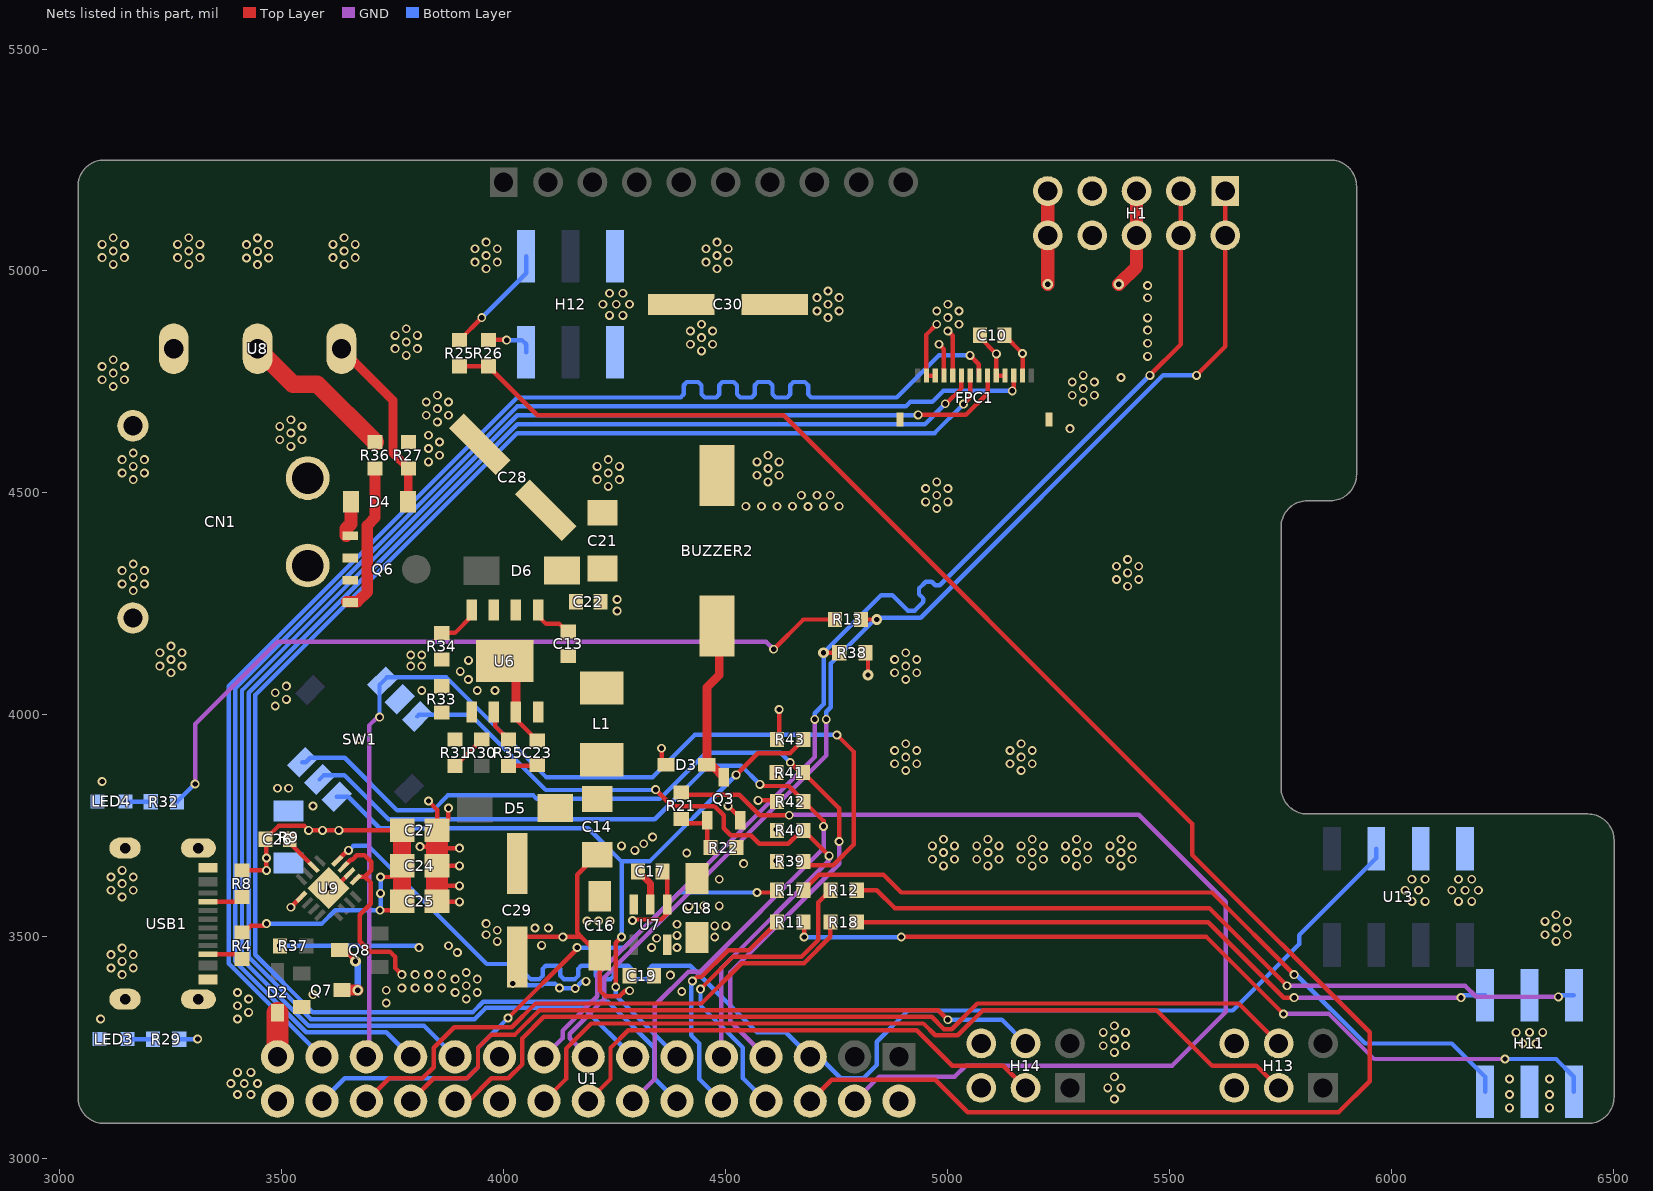
[diagram p0: the nets of this part, all layers, seen from the top]
# Altium PCB MISC51977.pcbdoc (part 2 of 4)
Units mil, origin at the board's own origin, x right, y up, seen from the top; angles counter-clockwise.
Board outline 3460 x 2170.19 mil, 4 copper layers (Top Layer, VCC, GND, Bottom Layer), stack 62.447 mil thick; 74 components, 60 nets, 282 pads, 462 vias.

## Via types
v1: diameter 20, hole 12, Top Layer to Bottom Layer, 455 vias
v2: diameter 24.02, hole 12, Top Layer to Bottom Layer, 7 vias

## Nets (pads, with @x,y where several pads share a name; then routed paths per layer and width w, separated by ;. In a path a pad name is that pad's centre, name@x,y a point inside that pad or via, vN(x,y) a via of type N, cw(c..) or ccw(c..) an arc to the next point about the centre after c; other vN are vias at no path point)
3V3: C10.2 C18.1 C19.1 FPC1.4 FPC1.10 FPC1.11 H1.5 H1.6 H1.9 H1.10 H13.5 H14.5 R13.2 R32.1 R38.2 R39.1 R40.1 R41.2 R42.2 R43.2 U7.5 | length 2550.2
  Top Layer w10: v1(4572.5,3807.5) 4611.88,3807.5 R42.2@4613.15,3808.77 ; v1(4607.56,4147.94) 4674.62,4215 R13.2@4745.34,4215 ; R43.2@4613.15,3941.94 4620.34,3949.13 4620.34,4012.78 v1(4620,4012.44) ; R38.2@4814.66,4140 4820,4134.66 v2(4820,4090) ; v1(4980,4835) 4991.1,4823.9 FPC1.4@4991.1,4764.22 ; C10.2@5072.44,4855 5072.44,4850 v1(5109.22,4813.23) FPC1.10@5109.22,4764.22 FPC1.11@5128.9,4764.22
  Top Layer w30: v2(5225,4970) H1.10@5225,5080 H1.9@5225,5180 ; v2(5385,4970) 5425,5010 H1.6@5425,5080 H1.5@5425,5180
  GND w10: v1(3304.54,3844.54) 3304.54,3979.54 3490,4165 4590.5,4165 v1(4607.56,4147.94)
  Bottom Layer w10: R32.1@3263.73,3804.54 3303.73,3844.54 v1(3304.54,3844.54)
  other v1: 4400.56,3376.99 4375,3414.02 4332.74,3475.98 4390,3475.98 4343.96,3497.01 4475,3500 4390,3503.59 4475,3525 4500,3525 4390,3528.56 4613.15,3671.94 4613.15,3741.94 4615,3866.94 5275,4645 5305,4705 5280,4720 5330,4720 5305,4735 5280,4750 5330,4750 5305,4765
$1N4144: CN1.2 D4.1 Q6.1 Q6.2 Q6.3 U8.3 | length 79.4
  Top Layer w30: Q6.1@3645.11,4405 3645.11,4420.11 3655.63,4430.63 D4.1@3655.63,4480
$1N4169: D4.2 R27.2 U8.1 | length 407.8
  Top Layer w20: U8.1@3633.97,4825 3750,4708.98 3750,4590.34 R27.2@3785,4555.34 3784.37,4554.71 D4.2@3784.37,4480
$1N4273: H11.2 R12.1 | length 1713.9
  Top Layer w10: R12.1@4794.66,3605.05 4839.95,3605.05 4880,3565 5589.02,3565 v1(5764.02,3390)
  GND w10: v1(5764.02,3390) 6165,3390 6190,3365 v1(6375,3365)
  Bottom Layer w10: v1(6375,3365) v1@6376.73,3363.27 ; v1@6378.27,3368.27 H11.2@6410,3368.27
$1N4282: R4.1 USB1.10 | length 80.9
  Top Layer w10: USB1.10@3333.51,3461.09 3399.24,3461.09 R4.1@3410,3450.34
$1N4283: R8.1 USB1.4 | length 80.9
  Top Layer w10: USB1.4@3333.51,3579.2 3399.34,3579.2 R8.1@3410,3589.87
$1N4817: BUZZER2.2 D3.2 Q3.3 | length 368.8
  Top Layer w20: BUZZER2.2@4485,4192.82 4485,4090 4457.38,4062.38 4457.38,3882.89 4472.1,3882.89 Q3.3@4495.26,3859.73
$1N4974: Q3.1 R21.2 R22.1 | length 120.6
  Top Layer w10: R21.2@4399.34,3755.8 4451.19,3755.8 Q3.1@4457.86,3762.48 4457.86,3713.16 R22.1@4464.92,3706.1
$1N5665: Q7.3 Q8.3 | length 146
  Top Layer w15: Q8.3@3635.63,3470 3644.48,3470 3665.69,3448.79 v2(3665.69,3445.39)
  Top Layer w25: Q7.3@3634.37,3380 v2(3670.69,3380)
  Bottom Layer w15: v2(3665.69,3445.39) 3670.69,3440.39 v2(3670.69,3380)
$1N14385: H11.1 R11.2 | length 1932
  Top Layer w10: R11.2@4674.66,3533.35 4676.3,3531.71 v1(4676.3,3499.64) ; v1(4895,3500) 5582.46,3500 v1(5755.98,3326.47)
  GND w10: v1(5755.98,3326.47) 5858.53,3326.47 5960,3225 v1(6255,3225)
  Bottom Layer w10: v1(4676.3,3499.64) 4894.64,3499.64 v1(4895,3500) ; v1(6255,3225) 6370,3225 6410,3185 H11.1@6410,3151.73
$1N14395: H11.6 R18.1 | length 1480.8
  Top Layer w10: R18.1@4794.66,3533.35 5586.65,3533.35 5756.73,3363.27 v1(5780,3363.27)
  GND w10: v1(5780,3363.27) v1(6155.98,3363.27)
  Bottom Layer w10: v1@6160.98,3368.27 H11.6@6210,3368.27
$1N14409: H11.5 R17.2 | length 1771.6
  Top Layer w10: R17.2@4674.66,3605.05 4709.61,3640 4855,3640 4895,3600 5595,3600 v1(5780,3415)
  Bottom Layer w10: v1(5780,3415) 5785,3415 5940,3260 6135,3260 6210,3185 H11.5@6210,3151.73
$1N22821: R36.1 U8.2 | length 352.1
  Top Layer w40: U8.2@3445,4825 3524.99,4745 3579.66,4745 R36.1@3710,4614.66
$1N23425: C26.1 U9.6 | length 85.1
  Top Layer w10: C26.1@3517.56,3720 3517.56,3711.36 U9.6@3571.59,3657.32
$1N29256: LED3.2 R29.1 | length 57.4
  Bottom Layer w10: LED3.2@3152.17,3269.92 3209.03,3269.92 R29.1@3209.41,3269.54
$1N41370: Q6.4 R36.2 | length 341.8
  Top Layer w25: Q6.4@3645.11,4255 3670,4255 3692.14,4277.14 3692.14,4427.14 3710,4445 R36.2@3710,4555.34
$1N45237: H12.6 R25.1 | length 250.7
  Top Layer w10: R25.1@3900,4844.66 3950,4894.66 v1(3950,4895)
  Bottom Layer w10: v1(3950,4895) 4050,4995 H12.6@4050,5033.27
$1N45238: H12.5 R26.1 | length 107.3
  Top Layer w10: R26.1@3965,4844.66 4005.77,4844.66 v1(4006.06,4844.37)
  Bottom Layer w10: v1(4006.06,4844.37) 4040.63,4844.37 4050,4835 H12.5@4050,4816.73
$2N1741: R34.2 U6.4 | length 96.4
  Top Layer w10: R34.2@3860,4184.66 3889.66,4184.66 3927.11,4222.11 U6.4@3927.11,4235.93
$2N1742: C21.2 C22.2 C28.1 D6.2 U6.2 U6.3
$2N1743: C13.2 U6.1 | length 95.6
  Top Layer w10: U6.1@4077.11,4235.93 4077.11,4222.89 4095,4205 4125,4205 4142.44,4187.56 C13.2@4145,4187.56
$2N1744: C13.1 L1.1 U6.8
$2N1746: C23.2 R35.1 | length 65.9
  Top Layer w10: R35.1@4010,3885.34 4072.9,3885.34 C23.2@4075,3887.44
$2N1747: R35.2 U6.6 | length 75.9
  Top Layer w10: U6.6@3977.11,4006.93 3980,4004.04 3980,3975 4010,3945 R35.2@4010,3944.66
$2N1748: R31.1 R33.2 U6.5
$2N1752: C14.2 C29.1 D5.1 L1.2
$2N1753: R30.1 R31.2 | length 84.6
  Top Layer w10: R31.2@3890,3885.34 3890.68,3885.34 R30.1@3950,3944.66
$2N1757: LED4.2 R32.2 | length 57.4
  Bottom Layer w10: LED4.2@3147.17,3804.92 3147.54,3804.54 R32.2@3204.41,3804.54
+5V: BUZZER2.1 C16.1 C17.1 C24.1 C25.1 C27.2 C30.1 D2.1 D3.1 Q7.2 R29.2 U1.29 U7.1 U7.3 U9.1 U9.3 U9.9 U13.7 | length 1386.8
  Top Layer w10: v1@3520,3565 v1(3520,3566.75) U9.9@3543.75,3590.51 ; U9.3@3638.36,3657.37 3655.01,3674.02 3658.69,3674.02 3668.69,3684.02 3685.98,3684.02 3700.86,3669.14 3700.86,3650.05 3686.67,3635.86 ; U9.1@3665,3629.53 U9.1@3666.2,3629.53 3672.53,3635.86 3686.67,3635.86 ; v1(3770,3415) 3755,3430 3755,3455 3742.93,3467.07 3697.93,3467.07 3675,3490 3675,3550 3700,3575 3700,3622.53 3686.67,3635.86 ; v1(3811,3703.43) 3848.37,3703.43 3849.37,3704.43 ; v1(3830,3805.98) 3849.37,3786.61 C27.2@3849.37,3740 3875,3765.63 v1(3875,3790) ; C25.1@3849.37,3580 3850.39,3578.98 v1(3900,3578.98) ; 3849.37,3615 v1(3900,3615) ; C24.1@3849.37,3660 v1(3900,3660) ; 3849.37,3710.63 3860,3700 v1(3900,3700) ; v1(4289.6,3536.98) 4291.9,3539.28 4354.28,3539.28 4367.4,3552.4 U7.1@4367.4,3573.04 4367.4,3637.78 C17.1@4357.56,3647.62 ; v1(4355,3925) 4355,3897.95 D3.1@4365.05,3887.89
  Top Layer w50: U1.29@3490,3230 D2.1@3490,3328.84 ; C25.1@3849.37,3580 3849.37,3615 C24.1@3849.37,3660 3849.37,3704.43 3849.37,3710.63 C27.2@3849.37,3740
  Bottom Layer w10: R29.2@3268.73,3269.54 3269.19,3270 v1(3310,3270)
  other v1: 3400,3315 3425,3330 3400,3345 3735,3350.98 3425,3360 3915,3360 3570,3370 3400,3375 3890,3375 3940,3375 3735,3380 3770,3385 3800,3385 3830,3385 3860,3385 3915,3390 3890,3405 3940,3405 3800,3415 3830,3415 3860,3415 3915,3420 4187.46,3536.06 4213.41,3536.06 4238.56,3536.06 6150,3580 6180,3580 6135,3605 6165,3605 6195,3605 6150,3630 6180,3630 4545,4470 4580,4470 4615,4470 4650,4470 4685,4469.59 4720,4470 4755,4470 4670,4495 4705,4495 4735,4495 4595,4525 4570,4540 4620,4540 4595,4555 4570,4570 4620,4570 4595,4585 4445,4820 4420,4835 4470,4835 4445,4850 4420,4865 4470,4865 4445,4880
AGND: C24.2 C25.2 C26.2 C27.1 R4.2 R8.2 R9.1 U9.2 U9.17 | length 1171.1
  Top Layer w10: R4.2@3410,3509.66 3414.66,3509.66 3430,3525 3460,3525 v1(3465,3530) ; R8.2@3410,3649.19 3410.81,3650 v1(3465,3650) v1(3465,3677.66) 3465,3717.44 C26.2@3462.44,3720 3492.44,3750 3550,3750 v1(3560,3740) v1(3591.39,3740) v1(3628.21,3740) C27.1@3770.63,3740 ; U9.17@3624.99,3610.01 3624.99,3616.15 U9.2@3652.28,3643.44 ; v1(3720.98,3560) 3750.63,3560 C25.2@3770.63,3580 ; v1(3722.15,3635) 3767.14,3635 3770.63,3631.51
  Top Layer w40: C25.2@3770.63,3580 3770.63,3631.51 C24.2@3770.63,3660 C27.1@3770.63,3740
  Bottom Layer w10: v1(3465,3530) 3590,3530 3620,3560 v1(3720.98,3560) 3722.15,3561.16 v1(3722.15,3598.06) v1(3722.15,3635)
  other v1: 3604.99,3610
BUZZER: R21.1 U1.4 | length 2496.7
  Top Layer w10: R21.1@4399.34,3815.12 4404.22,3820 4530,3820 4576,3774 v1(4642.81,3774)
  GND w10: v1(4642.81,3774) 4643.81,3775 5430,3775 5626.09,3578.91 5626.09,3331.09 5505,3210 5040,3210 5015,3185 4845,3185 U1.4@4790,3130
ENCODER_DIR_L: H13.3 U1.18 | length 1874.6
  Top Layer w10: U1.18@4090,3130 4140,3180 4140,3248.43 4196.57,3305 4945,3305 4971.69,3278.31 5022.41,3278.31 5079.11,3335 5470,3335 5595,3210 5695,3210 H13.3@5745,3160
ENCODER_DIR_R: H14.3 U1.16 | length 1146.1
  Top Layer w10: U1.16@4190,3130 4240,3180 4240,3250 4280,3290 4930,3290 5010,3210 5125,3210 H14.3@5175,3160
ENCODER_PWM_L: H13.4 U1.22 | length 2040.6
  Top Layer w10: U1.22@3890,3130 3920,3130 3971.61,3181.61 4010.04,3181.61 4041.61,3213.19 4041.61,3271.61 4090,3320 4963.63,3320 4991.31,3292.32 5008.69,3292.32 5066.37,3350 5655,3350 H13.4@5745,3260
ENCODER_PWM_R: H14.4 U1.24 | length 1526.4
  Top Layer w10: U1.24@3790,3130 3841.61,3181.61 3916.61,3181.61 3941.61,3206.61 3941.61,3250.04 3971.57,3280 4025,3280 4080,3335 4978.31,3335 v1(5000,3313.31)
  Bottom Layer w10: v1(5000,3313.31) 5121.69,3313.31 H14.4@5175,3260
GND: C10.1 C14.1 C16.2 C17.2 C18.2 C19.2 C21.1 C22.1 C23.1 C28.2 C29.2 C30.2 CN1.1 CN1.3 CN1.4 FPC1.2 FPC1.3 FPC1.5 FPC1.13 FPC1.15 FPC1.16 H1.7 H1.8 H11.3 H11.4 H12.1 H12.2 H13.6 H14.6 LED3.1 LED4.1 Q3.2 R9.2 R22.2 R27.1 R33.1 R34.1 R37.1 SW1.2 U1.2 U1.19 U1.20 U1.30 U6.7 U6.9 U7.2 U13.5 USB1.1 USB1.12 USB1.13 USB1.14 | length 1810.8
  Top Layer w10: v1(3495,3480) R37.1@3495.34,3480 R37.1@3495.68,3479.66 ; U6.7@4027.11,4006.93 4027.11,3990.45 C23.1@4075,3942.56 ; C29.2@4030,3449.88 4030,3500 v1(4132.83,3500) 4174.1,3500 ; C14.1@4210.19,3685.13 4165,3639.94 4165,3509.1 4174.1,3500 ; v1(4283.22,3378.65) 4273,3378.65 4260.52,3366.17 4228.83,3366.17 4215.49,3379.51 C16.2@4215.49,3458.61 4174.1,3500 ; v1(4505,3795) 4532.66,3767.34 Q3.2@4532.66,3762.48 ; FPC1.3@4971.41,4764.22 FPC1.2@4951.73,4764.22 4951.73,4856.73 v1(4975,4880) ; v1(5000,4865) 5010.78,4854.22 FPC1.5@5010.78,4764.22 ; C10.1@5127.56,4855 v1(5168.27,4814.3) FPC1.13@5168.27,4764.22
  Top Layer w15: C17.2@4302.44,3647.62 4330,3620.06 U7.2@4330,3573.04
  Top Layer w20: U6.9@4002.11,4121.43 4027.11,4096.43 U6.7@4027.11,4006.93
  Bottom Layer w10: v1(3495,3480) 3804.68,3480 v1(3808.82,3475.86) ; v1(4020,3395) 4050.18,3395 4054.19,3390.98 4085.81,3390.98 4089.82,3395 4115,3395 v1(4125,3385) 4125.98,3384.02 v1(4160.51,3384.02) 4176.5,3400 v1(4185,3400)
  other v1: 6265,3115 6355,3115 5375,3135 3400,3145 3430,3145 6265,3145 6355,3145.1 5360,3160 5390,3160 3385,3170 3415,3170 3445,3170 6265,3180 6355,3180 5375,3185 3400,3195 3430,3195 5375,3240 5350,3255 5400,3255 6295,3260 6325,3260 5375,3270 5350,3285 5400,3285 6280,3285 6310,3285 6340,3285 5375,3300 3091.69,3315 3140,3415 3115,3430 3165,3430 3140,3445 3115,3460 3165,3460 3895,3465 3140,3475 3875,3480 4085,3480.98 3985,3490 6370,3490 3960,3505 6345,3505 6395,3505 3985,3515 4070,3520 4100,3520 6370,3520 3960,3530 6345,3535 6395,3535 6370,3550 4416.93,3568.79 4450,3570 4485,3570 6045,3580 6075,3580 3140,3590 3115,3605 3165,3605 6030,3605 6060,3605 3140,3620 4485,3630 6045,3630 6075,3630 3115,3635 3165,3635 3140,3650 4990,3660 5090,3660 5190,3660 5290,3660 5390,3660 4540,3665 4965,3675 5015,3675 5065,3675 5115,3675 5165,3675 5215,3675 5265,3675 5315,3675 5365,3675 5415,3675 4411.71,3688.94 4990,3690 5090,3690 5190,3690 5290,3690 5390,3690 4295,3695 4265,3705 4965,3705 5015,3705 5065,3705 5115,3705 5165,3705 5215,3705 5265,3705 5315,3705 5365,3705 5415,3705 4315,3710 4990,3720 5090,3720 5190,3720 5290,3720 5390,3720 4335,3725 3570,3795 3490,3835 3515,3835 3095,3850 4905,3875 5165,3875 4880,3890 4930,3890 5140,3890 5190,3890 4905,3905 5165,3905 4880,3920 4930,3920 5140,3920 5190,3920 4905,3935 5165,3935 3675,3945 3485,4020 3510,4035 3485,4050 3815,4055 3940,4055 3980,4055 3510,4065 3920,4080 4905,4080 3250,4095 4880,4095 4930,4095 3901.72,4098.18 3225,4110 3275,4110 3790,4110 3815,4110 4905,4110 3920.15,4122.84 3250,4125 4880,4125 4930,4125 3790,4135 3815,4135 3225,4140 3275,4140 4905,4140 3250,4155 4255,4234.24 4255,4260 3165,4280 5405,4290 3140,4295 3190,4295 5380,4305 5430,4305 3165,4310 5405,4320 3140,4325 3190,4325 5380,4335 5430,4335 3165,4340 5405,4350 4975,4465 4950,4480 5000,4480 4975,4495 4950,4510 5000,4510 4235,4515 4975,4525 3165,4530 4210,4530 4260,4530 3140,4545 3190,4545 4235,4545 3165,4560 4210,4560 4260,4560 3830,4570 3140,4575 3190,4575 4235,4575 3855,4585 3165,4590 3830,4600 3520,4605 3855,4615 3495,4620 3545,4620 3830,4630 3520,4635 3495,4650 3545,4650 3850,4660 3520,4665 3825,4675 3875,4675 3850,4690 3825,4705 3875,4705 3850,4720 3120,4740 3095,4755 3145,4755 5390,4760 3120,4770 3095,4785 3145,4785 3120,4800 5450,4807.68 3780,4810 3755,4825 3805,4825 5450,4837.26 3780,4840 3755,4855 3805,4855 5450,4866.84 3780,4870 5025,4880 4730,4895 5000,4895 5450,4894.51 4237.89,4900 4267.89,4900 4705,4910 4755,4910 4975,4910 5025,4910 4222.89,4925 4252.89,4925 4282.89,4925 4730,4925 5000,4925 4705,4940 4755,4940 5450,4939.67 4237.89,4950 4267.89,4950 4730,4955 5450,4967.35 3960,5005 4480,5005 3445,5014.26 3120,5015 3290,5015 3640,5015 3935,5020 3985,5020 4455,5020 4505,5020 3420,5029.26 3470,5029.26 3095,5030 3145,5030 3265,5030 3315,5030 3615,5030 3665,5030 3960,5035 4480,5035 3445,5044.26 3120,5045 3290,5045 3640,5045 3935,5050 3985,5050 4455,5050 4505,5050 3420,5059.26 3470,5059.26 3095,5060 3145,5060 3265,5060 3315,5060 3615,5060 3665,5060 3960,5065 4480,5065 3445,5074.26 3120,5075 3290,5075 3640,5075
GOVERNOR: R25.2 R26.2 U1.6 | length 4161.9
  Top Layer w10: R25.2@3900,4785.34 R26.2@3965,4785.34 4075.34,4675 4630,4675 5550,3755 5550,3685 5950,3285 5950,3175 5880,3105 5045,3105 4971.61,3178.39 4738.39,3178.39 U1.6@4690,3130
I2C_SCL: H1.1 H1.2 R13.1 U1.15 | length 2717
  Top Layer w10: R13.1@4804.66,4215 v2(4839.53,4215) ; v1(5560,4765) 5625,4830 H1.2@5625,5080 H1.1@5625,5180
  GND w10: U1.15@4190,3230 4147.99,3272.01 4147.99,3282.01 4225.98,3360 4225.98,3408.7 4725.98,3908.7 v1(4725.98,3990) v1@4725.55,3990
  Bottom Layer w10: v1(4725.98,3990) 4725.98,4007.52 4735.98,4017.52 4735.98,4115.98 4839.02,4219.02 4938.69,4219.02 5484.68,4765 v1(5560,4765)
I2C_SDA: H1.3 H1.4 R38.1 U1.17 | length 2711.6
  Top Layer w10: v2(4720,4140) R38.1@4755.34,4140 ; v1(5455,4765) 5525,4835 H1.4@5525,5080 H1.3@5525,5180
  GND w10: U1.17@4090,3230 4132.01,3272.01 4132.01,3288.63 4210,3366.62 4210,3415.32 4700,3905.32 v1(4700,3990)
  Bottom Layer w10: v1(4700,3990) 4700,4004.14 4720,4024.14 v2(4720,4140) 4850,4270 4875,4270 4910,4235 4925,4235 4945,4255 4945,4262.16 4935,4272.16 4935,4285 4950,4300 4963.73,4300 4971.87,4291.87 4981.87,4291.87 v1(5455,4765)
KEY_DOWN: R43.1 SW1.4 U1.11 | length 1724.6
  Top Layer w10: v1(4251.83,3387.16) 4251.83,3419.31 4251.99,3419.46 4251.99,3486.99 v1(4265,3500) ; v1(4523.06,3865) 4572,3913.94 4644.48,3913.94 R43.1@4672.47,3941.94
  Bottom Layer w10: SW1.4@3623.51,3815.55 3649.45,3815.55 3720,3745 4190,3745 4265,3670 ; v1(4251.83,3387.16) 4251.83,3368.17 U1.11@4390,3230 ; v1(4265,3500) 4265,3670 ; v1(4523.06,3865) 4328.06,3670 4265,3670
KEY_LEFT: R40.2 SW1.3 U1.9 | length 1657.9
  Top Layer w10: v1(4341.74,3831.74) 4378.96,3794.52 4474.23,3794.52 4495,3773.75 4495,3745 4510.91,3729.09 4555.91,3729.09 4575,3710 4640.53,3710 4672.47,3741.94 4673.06,3741.94 v1(4732.5,3682.5)
  GND w10: U1.9@4490,3230 4490,3430 4732.5,3672.5 v1(4732.5,3682.5)
  Bottom Layer w10: SW1.3@3804.45,3996.5 3807.95,4000 3925,4000 4094.02,3830.98 4340.98,3830.98 v1(4341.74,3831.74)
KEY_MID: R42.1 SW1.5 U1.14 | length 2107.4
  Top Layer w10: v1(4576.38,3843.69) 4580.07,3840 4641.24,3840 4720,3761.24 v1(4720,3749.02)
  GND w10: U1.14@4290,3130 4340,3180 4340,3346.1 4415.76,3421.86 4442.18,3421.86 4720,3699.68 v1(4720,3749.02)
  Bottom Layer w10: SW1.5@3584.53,3854.53 3594.53,3864.53 3640.47,3864.53 3740,3765 4340,3765 4460.98,3885.98 4534.02,3885.98 v1@4576.31,3843.69
KEY_RIGHT: R41.1 SW1.6 U1.7 | length 2069.1
  Top Layer w10: v1(4645.01,3892.96) 4666.03,3871.94 4672.47,3871.94 4755,3789.41 v1(4755,3715)
  GND w10: U1.7@4590,3230 4510,3310 4510,3420 4755,3665 v1(4755,3715)
  Bottom Layer w10: SW1.6@3545.55,3893.5 3553.5,3893.5 3563.5,3903.5 3641.5,3903.5 3760,3785 3840,3785 3873.63,3818.63 4066.37,3818.63 4074.24,3810.76 4350.76,3810.76 4455,3915 4622.97,3915 v1(4645.01,3892.96)
KEY_UP: R39.2 SW1.1 U1.25 | length 2424.1
  Top Layer w10: R39.2@4672.47,3671.94 4682.89,3661.52 4741.52,3661.52 4787.5,3707.5 4787.5,3917.5 v1(4750,3955)
  GND w10: U1.25@3690,3230 3690,3235 3696.16,3241.16 3696.16,3976.16 3715,3995 v1(3720,3995)
  Bottom Layer w10: v1(3720,3995) 3719.7,3995.3 3719.7,4067.65 3736.5,4084.45 3870.55,4084.45 4095,3860 4335,3860 4430,3955 v1(4750,3955)
MOTOR_DIR_L: R12.2 U1.8 | length 748
  Top Layer w10: v1(4442.82,3382.5) 4442.82,3382.82 4515,3455 4670,3455 4708.48,3493.48 4708.48,3578.19 R12.2@4735.34,3605.05
  Bottom Layer w10: v1(4442.82,3382.5) 4442.82,3345.6 4538.39,3250.04 4538.39,3181.61 U1.8@4590,3130
MOTOR_DIR_R: R11.1 U1.10 | length 546.2
  Top Layer w10: v1(4424.45,3400.87) 4425.87,3400.87 4435,3410 4445,3410 4505,3470 4551.99,3470 R11.1@4615.34,3533.35
  Bottom Layer w10: v1(4424.45,3400.87) 4424.45,3394.39 4421.55,3391.49 4421.55,3278.38 4440,3259.92 4440,3180 U1.10@4490,3130
MOTOR_PWM_L: R18.2 U1.26 | length 1257.2
  Top Layer w10: U1.26@3690,3130 3741.61,3181.61 3816.61,3181.61 3841.61,3206.61 3841.61,3250.04 3888.15,3296.57 4017.88,3296.57 4071.31,3350 4445,3350 4535.98,3440.98 4675.98,3440.98 4735.34,3500.34 R18.2@4735.34,3533.35
MOTOR_PWM_R: R17.1 U1.28 | length 1249
  Top Layer w10: v1(4009.19,3317.56) 4165,3473.37 v1(4165,3475.98) ; v1(4570,3600) 4610.29,3600 R17.1@4615.34,3605.05
  Bottom Layer w10: U1.28@3590,3130 3641.61,3181.61 3916.61,3181.61 3941.61,3206.61 3941.61,3250.04 3969.96,3278.39 ; 3970.02,3278.39 v1(4009.19,3317.56) ; v1(4165,3475.98) 4270.98,3475.98 4395,3600 v1(4570,3600)
RX: U1.5 U9.4 U13.3 | length 3002.7
  Top Layer w10: U9.4@3624.45,3671.29 3648.16,3695 v1(3650,3695)
  Bottom Layer w10: v1(3650,3695) 3650.98,3695 3660.98,3705 3695,3705 3960.98,3439.02 4025.98,3439.02 4060,3405 4080,3405 4087.07,3412.07 4087.07,3427.93 4094.14,3435 4120,3435 4127.07,3427.93 4127.07,3412.93 4135,3405 4160,3405 4167.07,3412.07 4167.07,3427.93 4174.14,3435 4200,3435 4207.07,3427.93 4207.07,3412.93 4215,3405 4240,3405 4247.07,3412.07 4247.07,3427.93 4254.14,3435 4280,3435 4287.07,3427.93 4287.07,3412.93 4295,3405 4320,3405 4327.07,3412.07 4327.07,3427.93 4334.14,3435 4420,3435 4570,3285 4635,3285 U1.5@4690,3230 4710,3230 4758.39,3181.61 4810.04,3181.61 4840,3211.57 4840,3263.94 4910.36,3334.29 5641.69,3334.29 5791.09,3483.69 5791.09,3503.69 5965,3677.6 U13.3@5965,3698.27
TFFT180_SDA: FPC1.8 U1.27 | length 3168.3
  Top Layer w10: v1(5050,4810) 5069.85,4790.15 FPC1.8@5069.85,4764.22
  Bottom Layer w10: U1.27@3590,3230 3380,3440 3380,4065 4030,4715 4397.93,4715 4405,4722.07 4405,4742.93 4412.07,4750 4437.93,4750 4445,4742.93 4445,4722.07 4452.07,4715 4477.93,4715 4485,4722.07 4485,4742.93 4492.07,4750 4517.93,4750 4525,4742.93 4525,4722.07 4532.07,4715 4557.93,4715 4565,4722.07 4565,4742.93 4572.07,4750 4597.93,4750 4605,4742.93 4605,4722.07 4612.07,4715 4637.93,4715 4645,4722.07 4645,4742.93 4652.07,4750 4677.93,4750 4685,4742.93 4685,4722.07 4692.07,4715 4885,4715 4980,4810 v1(5050,4810)
TFT180_CS: FPC1.12 U1.23 | length 3162.4
  Top Layer w10: v1(5145,4730) 5148.59,4733.59 FPC1.12@5148.59,4764.22
  Bottom Layer w10: U1.23@3790,3230 3735,3285 3554.82,3285 3395,3444.82 3395,4060 4030,4695 4905,4695 4915,4705 4965,4705 4990,4730 v1(5145,4730)
TFT180_DC: FPC1.7 U1.12 | length 3668.6
  Top Layer w10: v1(5035,4700) 5050.15,4715.15 FPC1.7@5050.15,4764.22
  Bottom Layer w10: U1.12@4390,3130 4338.39,3181.61 4338.39,3250.04 4234.41,3354.02 3953.41,3354.02 3929.39,3330 3569.83,3330 3440,3459.83 3440,4045 4030,4635 4970,4635 v1(5035,4700)
TFT180_RES: FPC1.6 U1.13 | length 3492.1
  Top Layer w10: v1(4994.13,4700.87) 4995.87,4700.87 5030.48,4735.48 FPC1.6@5030.48,4764.22
  Bottom Layer w10: U1.13@4290,3230 4180,3340 3959.21,3340 3934.21,3315 3565,3315 3425,3455 3425,4050 4030,4655 4948.25,4655 v1(4994.13,4700.87)
TFT180_SCL: FPC1.9 U1.21 | length 3172.6
  Top Layer w10: v1(4933.03,4675.98) 5040.66,4675.98 5089.52,4724.85 FPC1.9@5089.52,4764.22
  Bottom Layer w10: U1.21@3890,3230 3820,3300 3560,3300 3410,3450 3410,4055.18 4029.82,4675 4932.05,4675 v1(4933.03,4675.98)